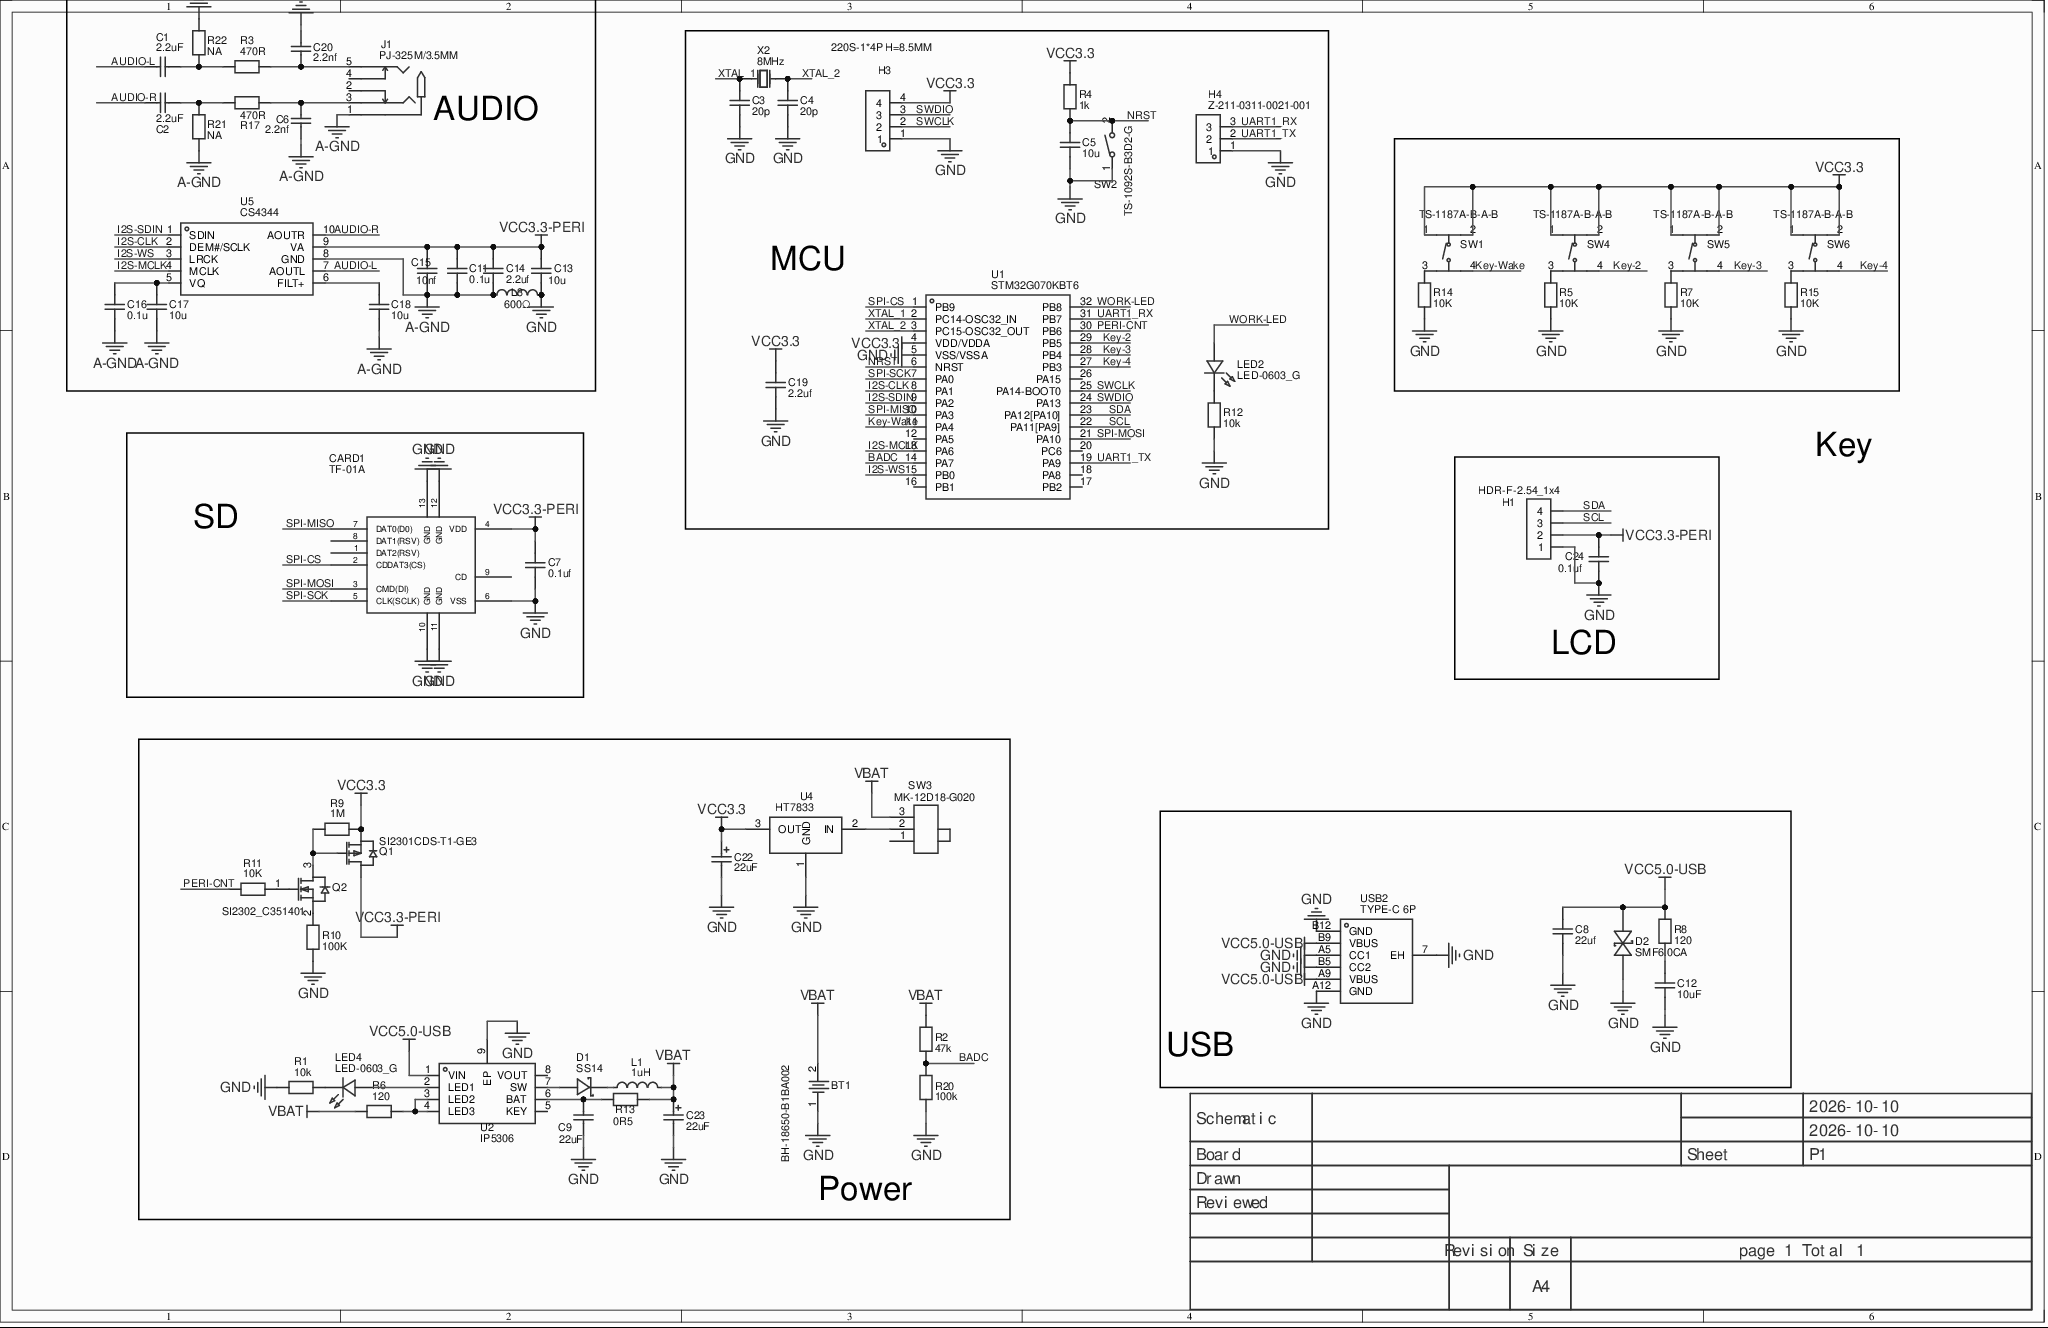
[diagram p0: MISC82317-2.schdoc]
# Altium schematic sheet MISC82317-2.schdoc
size 432 x 279 mm; Version: V1.0; @Project Name: MISC82317; @Update Date: 2026-10-10; @Create Date: 2026-10-10; @Board Name: MISC82317; @Create Time: 16:29:33; @Page Count: 1; @Page No: 1; @Schematic Name: MISC82317; @Update Time: 16:29:33; Size: A4

## Parts
BT1  BH-18650-B1BA002  [BATTERY-SMD_18650-1S-L77.1-W20.7-1]
C1  2.2uF  [C0603]
C2  2.2uF  [C0603]
C3  20p  [C0603]
C4  20p  [C0603]
C5  10u  [C0603]
C6  2.2nf  [C0603]
C7  0.1uf  [C0603]
C8  22uf  [C0603]
C9  22uF  [C0603]
C11  0.1u  [C0603]
C12  10uF  [C0603]
C13  10u  [C0603]
C14  2.2uf  [C0603]
C15  10nf  [C0603]
C16  0.1u  [C0603]
C17  10u  [C0603]
C18  10u  [C0603]
C19  2.2uf  [C0603]
C20  2.2nf  [C0603]
C22  22uF  [CAP-SMD_L3.5-W2.8-R-RD]
C23  22uF  [CAP-SMD_L3.5-W2.8-R-RD]
C24  0.1uf  [C0603]
CARD1  TF-01A  [TF-SMD_TF-01A]
D1  SS14  [SMA_L4.2-W2.6-LS5.3-RD]
D2  SMF6.0CA  [SOD-123FL_L2.8-W1.8-LS3.7-BI]
H1  HDR-F-2.54_1x4  [HDR-F-2.54_1X4]
H3  220S-1*4P H=8.5MM  [HDR-TH_4P-P2.54-V-F]
H4  Z-211-0311-0021-001  [HDR-TH_3P-P2.54-V-M-1]
J1  PJ-325M/3.5MM  [AUDIO-TH_PJ-325C]
L1  1uH  [IND-SMD_L6.8-W6.8_SMMS0630]
L3  600Ω  [L1206]
LED2  LED-0603_G  [LED0603_GREEN]
LED4  LED-0603_G  [LED0603_GREEN]
Q1  SI2301CDS-T1-GE3  [SOT-23-3_L3.0-W1.7-P0.95-LS2.9-BR]
Q2  SI2302_C351401  [SOT-23-3_L2.9-W1.3-P1.90-LS2.4]
R1  10k  [R0603]
R2  47k  [R0603]
R3  470R  [R0603]
R4  1k  [R0603]
R5  10K  [R0603]
R6  120  [R0603]
R7  10K  [R0603]
R8  120  [R0603]
R9  1M  [R0603]
R10  100K  [R0603]
R11  10K  [R0603]
R12  10k  [R0603]
R13  0R5  [R1206]
R14  10K  [R0603]
R15  10K  [R0603]
R17  470R  [R0603]
R20  100k  [R0603]
R21  NA  [R0603]
R22  NA  [R0603]
SW1  TS-1187A-B-A-B  [SW-SMD_4P-L5.1-W5.1-P3.70-LS6.5-TL-2]
SW2  TS-1092S-B3D2-G  [SW-SMD_L6.1-W3.6-LS7.9]
SW3  MK-12D18-G020  [SW-TH_MK-12D18-G040]
SW4  TS-1187A-B-A-B  [SW-SMD_4P-L5.1-W5.1-P3.70-LS6.5-TL-2]
SW5  TS-1187A-B-A-B  [SW-SMD_4P-L5.1-W5.1-P3.70-LS6.5-TL-2]
SW6  TS-1187A-B-A-B  [SW-SMD_4P-L5.1-W5.1-P3.70-LS6.5-TL-2]
U1  STM32G070KBT6  [LQFP-32_L7.0-W7.0-P0.80-LS9.0-BL]
U2  IP5306  [ESOP-8_L4.9-W3.9-P1.27-LS6.0-BL-EP]
U4  HT7833  [SOT-89_L4.5-W2.5-P1.50-LS4.2-BR]
U5  CS4344  [TSSOP-10_L3.0-W3.0-P0.50-LS4.9-BL]
USB2  TYPE-C 6P  [TYPE-C-SMD_TYPE-C-6P]
X2  8MHz  [CRYSTAL-SMD_L5.0-W3.2]

## Blocks framed on the sheet
AUDIO: C1 C2 C6 C11 C13-C18 C20 J1 L3 R3 R17 R21 R22 U5
MCU: C3-C5 C19 H3 H4 LED2 R4 R12 SW2 U1 X2
SD: C7 CARD1
LCD: C24 H1
Power: BT1 C9 C22 C23 D1 L1 LED4 Q1 Q2 R1 R2 R6 R9-R11 R13 R20 SW3 U2 U4
USB: C8 C12 D2 R8 USB2

## Nets
A-GND: C6.1 C11.1 C14.1 C15.1 C16.1 C17.1 C18.1 C20.2 J1.1 L3.1 R21.2 R22.1 U5.8(GND)
GND: BT1.1 C3.1 C4.1 C5.1 C7.1 C8.1 C9.1 C12.1 C13.1 C19.1 C22.2 C23.2 C24.1 CARD1.6(VSS) CARD1.10(GND) CARD1.11(GND) CARD1.12(GND) CARD1.13(GND) D2.1 H1.1 H3.1 H4.1 L3.2 R1.2 R5.1 R7.1 R10.2 R12.1 R14.1 R15.1 R20.1 SW2.1 U1.5(VSS/VSSA) U2.9(EP) U4.1(GND) USB2.7(EH) USB2.A5(CC1) USB2.A12(GND) USB2.B5(CC2) USB2.B12(GND)
VBAT: BT1.2 C23.1 L1.2 R2.2 R6.2 R13.2 SW3.3
VCC3.3: C19.2 C22.1 H3.4 Q1.2(S) R4.2 R9.1 SW1.1(A) SW1.2(B) SW4.1(A) SW4.2(B) SW5.1(A) SW5.2(B) SW6.1(A) SW6.2(B) U1.4(VDD/VDDA) U4.3(OUT)
VCC3.3-PERI: C7.2 C11.2 C13.2 C14.2 C15.2 C24.2 CARD1.4(VDD) H1.2 Q1.3(D) U5.9(VA)
VCC5.0-USB: C8.2 D2.2 R8.1 U2.1(VIN) USB2.A9(VBUS) USB2.B9(VBUS)
AUDIO-L: C1.1 U5.7(AOUTL)
AUDIO-R: C2.1 U5.10(AOUTR)
BADC: R2.1 R20.2 U1.14(PA7)
I2S-CLK: U1.8(PA1) U5.2(DEM#/SCLK)
I2S-MCLK: U1.13(PA6) U5.4(MCLK)
I2S-SDIN: U1.9(PA2) U5.1(SDIN)
I2S-WS: U1.15(PB0) U5.3(LRCK)
Key-2: SW4.4(D) U1.29(PB5)
Key-3: SW5.4(D) U1.28(PB4)
Key-4: SW6.4(D) U1.27(PB3)
Key-Wake: SW1.4(D) U1.11(PA4)
NRST: C5.2 R4.1 SW2.2 U1.6(NRST)
PERI-CNT: R11.1 U1.30(PB6)
SCL: H1.3 U1.22(PA11[PA9])
SDA: H1.4 U1.23(PA12[PA10])
SPI-CS: CARD1.2(CDDAT3(CS)) U1.1(PB9)
SPI-MISO: CARD1.7(DAT0(D0)) U1.10(PA3)
SPI-MOSI: CARD1.3(CMD(DI)) U1.21(PA10)
SPI-SCK: CARD1.5(CLK(SCLK)) U1.7(PA0)
SWCLK: H3.2 U1.25(PA14-BOOT0)
SWDIO: H3.3 U1.24(PA13)
UART1_RX: H4.3 U1.31(PB7)
UART1_TX: H4.2 U1.19(PA9)
WORK-LED: LED2.1 U1.32(PB8)
XTAL_1: C3.2 U1.2(PC14-OSC32_IN) X2.1(OSC1)
XTAL_2: C4.2 U1.3(PC15-OSC32_OUT) X2.2(OSC2)
NetC1_2: C1.2 R3.2 R22.2
NetC2_2: C2.2 R17.2 R21.1
NetC6_2: C6.2 J1.3 R17.1
NetC9_2: C9.2 R13.1 U2.6(BAT)
NetC12_2: C12.2 R8.2
NetC16_2: C16.2 C17.2 U5.5(VQ)
NetC18_2: C18.2 U5.6(FILT+)
NetC20_1: C20.1 J1.5 R3.1
NetD1_1: D1.1(K) L1.1
NetD1_2: D1.2(A) U2.7(SW)
NetLED2_2: LED2.2 R12.2
NetLED4_1: LED4.1 U2.2(LED1)
NetLED4_2: LED4.2 R1.1
NetQ1_1: Q1.1(G) Q2.3(D) R9.2
NetQ2_1: Q2.1(G) R11.2
NetQ2_2: Q2.2(S) R10.1
NetR5_2: R5.2 SW4.3(C)
NetR6_1: R6.1 U2.3(LED2) U2.4(LED3)
NetR7_2: R7.2 SW5.3(C)
NetR14_2: R14.2 SW1.3(C)
NetR15_2: R15.2 SW6.3(C)
NetSW3_2: SW3.2 U4.2(IN)

Not connected (* = marked no-connect by the designer): CARD1 1(DAT2(RSV))* 8(DAT1(RSV))* 9(CD)*; J1 2* 4*; SW3 1*; U1 12(PA5)* 16(PB1)* 17(PB2)* 18(PA8)* 20(PC6)* 26(PA15)*; U2 5(KEY)* 8(VOUT)*

## Notes on the sheet
- Key
- 2026-10-10
- Schematic
- Board
- Sheet
- P1
- Drawn
- Reviewed
- Revision
- Size
- A4
- page 1 Total 1

## Library data of the parts
BT1 = BH-18650-B1BA002: Manufacturer: MYOUNG(美阳); Add into BOM: yes; 3D Model: 6c4af93ff24747e7be32603ea977d5150819f05c4eef4c71ace90d822a990e87; Symbol: BH-18650-B1BA002; Device: BH-18650-B1BA002; Convert to PCB: yes; Supplier: LCSC; Supplier Part: C2988620; Manufacturer Part: BH-18650-B1BA002; link: https://atta.szlcsc.com/upload/public/pdf/source/20220402/870DB99AB50CA0DF8D51CF7C86A51FAB.pdf; JLCPCB Part Class: Extended Part; Origin Footprint: BATTERY-SMD_18650-1S-L77.1-W20.7-1; FootprintName: BATTERY-SMD_18650-1S-L77.1-W20.7-1; ModelName: BATTERY-SMD_18650-1S-L77.1-W20.7-1
C1 C2 C6 C20 = CL10A225KO8NNNC: Manufacturer: SAMSUNG; Add into BOM: yes; 3D Model: fca5be93b99f4b5a9a2fd372d58c31d90819f05c4eef4c71ace90d822a990e87; Device: CL10A225KO8NNNC; Convert to PCB: yes; Supplier: LCSC; Manufacturer Part: CL10A225KO8NNNC; Supplier Part: C23630; JLCPCB Part Class: Basic Part; Origin Footprint: C0603; FootprintName: C0603; ModelName: C0603
  C1 C2: Symbol: 2.2uF
  C6 C20: Symbol: 2.2nf
C3 C4 = 20p: Add into BOM: yes; 3D Model: fca5be93b99f4b5a9a2fd372d58c31d90819f05c4eef4c71ace90d822a990e87; Symbol: 20p; Device: 20p; Convert to PCB: yes; Origin Footprint: C0603; FootprintName: C0603; ModelName: C0603
C5 C13 C17 C18 = 10u: Add into BOM: yes; 3D Model: fca5be93b99f4b5a9a2fd372d58c31d90819f05c4eef4c71ace90d822a990e87; Symbol: 10u; Device: 10u; Convert to PCB: yes; Origin Footprint: C0603; FootprintName: C0603; ModelName: C0603
C7 C24 = 0.1uf: Add into BOM: yes; 3D Model: fca5be93b99f4b5a9a2fd372d58c31d90819f05c4eef4c71ace90d822a990e87; Symbol: 0.1uf; Device: 0.1uf; Convert to PCB: yes; Origin Footprint: C0603; FootprintName: C0603; ModelName: C0603
C8 C12 = 0603X106M250NT: Manufacturer: FH(Guangdong Fenghua Advanced Tech); Add into BOM: yes; 3D Model: fca5be93b99f4b5a9a2fd372d58c31d90819f05c4eef4c71ace90d822a990e87; Device: 0603X106M250NT; Convert to PCB: yes; Supplier: LCSC; Supplier Part: C479655; Manufacturer Part: 0603X106M250NT; JLCPCB Part Class: Extended Part; Origin Footprint: C0603; FootprintName: C0603; ModelName: C0603
  C8: Symbol: 22uf
  C12: Symbol: 10uF
C9 = CC0603MRX5R5BB226: Manufacturer: YAGEO; Add into BOM: yes; 3D Model: fca5be93b99f4b5a9a2fd372d58c31d90819f05c4eef4c71ace90d822a990e87; Symbol: 22uF; Device: CC0603MRX5R5BB226; Convert to PCB: yes; Supplier: LCSC; Manufacturer Part: CC0603MRX5R5BB226; Supplier Part: C109448; JLCPCB Part Class: Extended Part; Origin Footprint: C0603; FootprintName: C0603; ModelName: C0603
C11 C16 = 0.1u: Add into BOM: yes; 3D Model: fca5be93b99f4b5a9a2fd372d58c31d90819f05c4eef4c71ace90d822a990e87; Symbol: 0.1u; Device: 0.1u; Convert to PCB: yes; Origin Footprint: C0603; FootprintName: C0603; ModelName: C0603
C14 C19 = 2.2uf: Add into BOM: yes; 3D Model: fca5be93b99f4b5a9a2fd372d58c31d90819f05c4eef4c71ace90d822a990e87; Symbol: 2.2uf; Device: 2.2uf; Convert to PCB: yes; Origin Footprint: C0603; FootprintName: C0603; ModelName: C0603
C15 = 10nf: Add into BOM: yes; 3D Model: fca5be93b99f4b5a9a2fd372d58c31d90819f05c4eef4c71ace90d822a990e87; Symbol: 10nf; Device: 10nf; Convert to PCB: yes; Origin Footprint: C0603; FootprintName: C0603; ModelName: C0603
C22 C23 = TAJB226K016RNJ: Manufacturer: AVX; Add into BOM: yes; Symbol: 22uF; Device: TAJB226K016RNJ; Convert to PCB: yes; Supplier: LCSC; Manufacturer Part: TAJB226K016RNJ; Supplier Part: C8020; JLCPCB Part Class: Extended Part; Origin Footprint: CAP-SMD_L3.5-W2.8-R-RD; FootprintName: CAP-SMD_L3.5-W2.8-R-RD
CARD1 = TF-01A: Manufacturer: HRO; Add into BOM: yes; 3D Model: 2d64e7db065c4e679bbb440594759bbc0819f05c4eef4c71ace90d822a990e87; Symbol: TF-01A; Device: TF-01A; Convert to PCB: yes; Supplier: LCSC; Manufacturer Part: TF-01A; Supplier Part: C91145; JLCPCB Part Class: Extended Part; Origin Footprint: TF-SMD_TF-01A; FootprintName: TF-SMD_TF-01A; ModelName: TF-SMD_TF-01A
D1 = SS14: Manufacturer: MDD; Add into BOM: yes; 3D Model: c9e8185d46a94015b9fa58a531b156cf0819f05c4eef4c71ace90d822a990e87; Symbol: SS14; Device: SS14; Convert to PCB: yes; Supplier: LCSC; Manufacturer Part: SS14; Supplier Part: C2480; JLCPCB Part Class: Basic Part; Origin Footprint: SMA_L4.2-W2.6-LS5.3-RD; FootprintName: SMA_L4.2-W2.6-LS5.3-RD; ModelName: SMA_L4.2-W2.6-LS5.3-RD
D2 = SMF6.0CA: Manufacturer: MDD; Add into BOM: yes; 3D Model: d105299b3871451c86f679efef28ff8f0819f05c4eef4c71ace90d822a990e87; Symbol: SMF6.0CA; Device: SMF6.0CA; Convert to PCB: yes; Supplier: LCSC; Manufacturer Part: SMF6.0CA; Supplier Part: C123791; JLCPCB Part Class: Extended Part; Origin Footprint: SOD-123FL_L2.8-W1.8-LS3.7-BI; FootprintName: SOD-123FL_L2.8-W1.8-LS3.7-BI; ModelName: SOD-123FL_L2.8-W1.8-LS3.7-BI
H1 = HDR-F-2.54_1x4: Add into BOM: yes; 3D Model: f101a8d78d1e4ea1b9dbaf5a3cdaf2060819f05c4eef4c71ace90d822a990e87; Symbol: HDR-F-2.54_1x4; Device: HDR-F-2.54_1x4; Convert to PCB: yes; Supplier Part: C225501; Supplier: LCSC; Origin Footprint: HDR-F-2.54_1X4; FootprintName: HDR-F-2.54_1X4; ModelName: HDR-F-2.54_1x4
H3 = 220S-1*4P H=8.5MM Ytype Gold-plated: Manufacturer: Ckmtw; Add into BOM: yes; 3D Model: d187812051054f85879fcaa51a310d8e0819f05c4eef4c71ace90d822a990e87; Symbol: 220S-1*4P H=8.5MM; Device: 220S-1*4P H=8.5MM Ytype Gold-plated; Convert to PCB: yes; Supplier: LCSC; Manufacturer Part: 220S-1*4P H=8.5MM Ytype Gold-plated; Supplier Part: C124413; JLCPCB Part Class: Extended Part; Origin Footprint: HDR-TH_4P-P2.54-V-F; FootprintName: HDR-TH_4P-P2.54-V-F; ModelName: HDR-TH_4P-P2.54-V-F
H4 = Z-211-0311-0021-001: Manufacturer: ZHENGLING; Add into BOM: yes; Symbol: Z-211-0311-0021-001; Device: Z-211-0311-0021-001; Convert to PCB: yes; Supplier: LCSC; Manufacturer Part: Z-211-0311-0021-001; Supplier Part: C152153; JLCPCB Part Class: Extended Part; Origin Footprint: HDR-TH_3P-P2.54-V-M-1; FootprintName: HDR-TH_3P-P2.54-V-M-1
J1 = PJ-325M/3.5MM: Manufacturer: BOOMELE; Add into BOM: yes; 3D Model: 332d8d5c7f544556a9ac40ab7a6b8b0c0819f05c4eef4c71ace90d822a990e87; Symbol: PJ-325M/3.5MM; Device: PJ-325M/3.5MM; Convert to PCB: yes; Supplier: LCSC; Manufacturer Part: PJ-325M/3.5MM; Supplier Part: C26230; JLCPCB Part Class: Extended Part; Origin Footprint: AUDIO-TH_PJ-325C; FootprintName: AUDIO-TH_PJ-325C; ModelName: AUDIO-TH_PJ-325C
L1 = SMMS0630-1R0M: Manufacturer: SXN; Add into BOM: yes; Symbol: 1uH; Device: SMMS0630-1R0M; Convert to PCB: yes; Supplier: LCSC; Manufacturer Part: SMMS0630-1R0M; Supplier Part: C128684; JLCPCB Part Class: Extended Part; Origin Footprint: IND-SMD_L6.8-W6.8_SMMS0630; FootprintName: IND-SMD_L6.8-W6.8_SMMS0630
L3 = CBW321609U601T: Manufacturer: FH; Add into BOM: yes; Symbol: 600Ω; Device: CBW321609U601T; Convert to PCB: yes; Supplier: LCSC; Manufacturer Part: CBW321609U601T; Supplier Part: C73732; JLCPCB Part Class: Extended Part; Origin Footprint: L1206; FootprintName: L1206
LED2 LED4 = 19-217/GHC-YR1S2/3T: Manufacturer: EVERLIGHT(台湾亿光); Add into BOM: yes; Symbol: LED-0603_G; Device: 19-217/GHC-YR1S2/3T; Convert to PCB: yes; Manufacturer Part: 19-217/GHC-YR1S2/3T; Supplier Part: C72043; Supplier: LCSC; Origin Footprint: LED0603_GREEN; FootprintName: LED0603_GREEN
Q1 = SI2301CDS-T1-GE3: Manufacturer: VISHAY; Add into BOM: yes; Symbol: SI2301CDS-T1-GE3; Device: SI2301CDS-T1-GE3; Convert to PCB: yes; Supplier: LCSC; Manufacturer Part: SI2301CDS-T1-GE3; Supplier Part: C10487; JLCPCB Part Class: Basic Part; Origin Footprint: SOT-23-3_L3.0-W1.7-P0.95-LS2.9-BR; FootprintName: SOT-23-3_L3.0-W1.7-P0.95-LS2.9-BR
Q2 = SI2302: Manufacturer: PUOLOP; Add into BOM: yes; 3D Model: 115ef394a879442d90491e61279301380819f05c4eef4c71ace90d822a990e87; Symbol: SI2302_C351401; Device: SI2302; Convert to PCB: yes; Supplier: LCSC; Supplier Part: C351401; Manufacturer Part: SI2302; JLCPCB Part Class: Extended Part; Origin Footprint: SOT-23-3_L2.9-W1.3-P1.90-LS2.4; FootprintName: SOT-23-3_L2.9-W1.3-P1.90-LS2.4; ModelName: SOT-23-3_L2.9-W1.3-P1.90-LS2.4
R1 R12 = 10k: Add into BOM: yes; 3D Model: fc143cca1e79419f9cd78b61e9279f080819f05c4eef4c71ace90d822a990e87; Symbol: 10k; Device: 10k; Convert to PCB: yes; Origin Footprint: R0603; FootprintName: R0603; ModelName: R0603
R2 = 47k: Add into BOM: yes; 3D Model: fc143cca1e79419f9cd78b61e9279f080819f05c4eef4c71ace90d822a990e87; Symbol: 47k; Device: 47k; Convert to PCB: yes; Origin Footprint: R0603; FootprintName: R0603; ModelName: R0603
R3 R17 = 470R: Add into BOM: yes; 3D Model: fc143cca1e79419f9cd78b61e9279f080819f05c4eef4c71ace90d822a990e87; Symbol: 470R; Device: 470R; Convert to PCB: yes; Origin Footprint: R0603; FootprintName: R0603; ModelName: R0603
R4 = 1k: Add into BOM: yes; 3D Model: fc143cca1e79419f9cd78b61e9279f080819f05c4eef4c71ace90d822a990e87; Symbol: 1k; Device: 1k; Convert to PCB: yes; Origin Footprint: R0603; FootprintName: R0603; ModelName: R0603
R5 R7 R11 R14 R15 = 10K: Add into BOM: yes; 3D Model: fc143cca1e79419f9cd78b61e9279f080819f05c4eef4c71ace90d822a990e87; Symbol: 10K; Device: 10K; Convert to PCB: yes; Origin Footprint: R0603; FootprintName: R0603; ModelName: R0603
R6 R8 = 120: Add into BOM: yes; 3D Model: fc143cca1e79419f9cd78b61e9279f080819f05c4eef4c71ace90d822a990e87; Symbol: 120; Device: 120; Convert to PCB: yes; Origin Footprint: R0603; FootprintName: R0603; ModelName: R0603
R9 = 1M: Add into BOM: yes; 3D Model: fc143cca1e79419f9cd78b61e9279f080819f05c4eef4c71ace90d822a990e87; Symbol: 1M; Device: 1M; Convert to PCB: yes; Origin Footprint: R0603; FootprintName: R0603; ModelName: R0603
R10 = 100K: Add into BOM: yes; 3D Model: fc143cca1e79419f9cd78b61e9279f080819f05c4eef4c71ace90d822a990e87; Symbol: 100K; Device: 100K; Convert to PCB: yes; Origin Footprint: R0603; FootprintName: R0603; ModelName: R0603
R13 = 1206W4F590LT5E: Manufacturer: UNI-ROYAL(Uniroyal Elec); Add into BOM: yes; Resistance (Ohms): 0.59; Symbol: 0R5; Device: 1206W4F590LT5E; Convert to PCB: yes; Supplier: LCSC; Supplier Part: C473018; Manufacturer Part: 1206W4F590LT5E; JLCPCB Part Class: Extended Part; Origin Footprint: R1206; FootprintName: R1206
R20 = 100k: Add into BOM: yes; 3D Model: fc143cca1e79419f9cd78b61e9279f080819f05c4eef4c71ace90d822a990e87; Symbol: 100k; Device: 100k; Convert to PCB: yes; Origin Footprint: R0603; FootprintName: R0603; ModelName: R0603
R21 R22 = NA: Add into BOM: yes; 3D Model: fc143cca1e79419f9cd78b61e9279f080819f05c4eef4c71ace90d822a990e87; Symbol: NA; Device: NA; Convert to PCB: yes; Origin Footprint: R0603; FootprintName: R0603; ModelName: R0603
SW1 SW4-SW6 = TS-1187A-B-A-B: Manufacturer: XKB Enterprise; Add into BOM: yes; Symbol: TS-1187A-B-A-B; Device: TS-1187A-B-A-B; Convert to PCB: yes; Supplier: LCSC; Supplier Part: C318884; Manufacturer Part: TS-1187A-B-A-B; JLCPCB Part Class: Basic Part; Origin Footprint: SW-SMD_4P-L5.1-W5.1-P3.70-LS6.5-TL-2; FootprintName: SW-SMD_4P-L5.1-W5.1-P3.70-LS6.5-TL-2
SW2 = TS-1092S-B3D2-G: Manufacturer: Yuandi; Add into BOM: yes; Symbol: TS-1092S-B3D2-G; Device: TS-1092S-B3D2-G; Convert to PCB: yes; Supplier: LCSC; Supplier Part: C520860; Manufacturer Part: TS-1092S-B3D2-G; JLCPCB Part Class: Extended Part; Origin Footprint: SW-SMD_L6.1-W3.6-LS7.9; FootprintName: SW-SMD_L6.1-W3.6-LS7.9
SW3 = MK-12D18-G020: Manufacturer: G-Switch(品赞); Add into BOM: yes; 3D Model: 10e91de5902f4d769c8626292907b3900819f05c4eef4c71ace90d822a990e87; Symbol: MK-12D18-G020; Device: MK-12D18-G020; Convert to PCB: yes; Supplier: LCSC; Supplier Part: C3019727; Manufacturer Part: MK-12D18-G020; link: https://atta.szlcsc.com/upload/public/pdf/source/20201201/C963202_825FB742C5BA766BED52E1DDA96DE5A3.pdf; Origin Footprint: SW-TH_MK-12D18-G040; FootprintName: SW-TH_MK-12D18-G040; ModelName: SW-TH_MK-12D18-G040
U1 = STM32G070KBT6: Manufacturer: STMicroelectronics; Add into BOM: yes; Symbol: STM32G070KBT6; Device: STM32G070KBT6; Convert to PCB: yes; Supplier: LCSC; Supplier Part: C529339; Manufacturer Part: STM32G070KBT6; JLCPCB Part Class: Extended Part; Origin Footprint: LQFP-32_L7.0-W7.0-P0.80-LS9.0-BL; FootprintName: LQFP-32_L7.0-W7.0-P0.80-LS9.0-BL
U2 = IP5306: Manufacturer: INJOINIC; Add into BOM: yes; Symbol: IP5306; Device: IP5306; Convert to PCB: yes; Supplier: LCSC; Supplier Part: C181692; Manufacturer Part: IP5306; JLCPCB Part Class: Extended Part; Origin Footprint: ESOP-8_L4.9-W3.9-P1.27-LS6.0-BL-EP; FootprintName: ESOP-8_L4.9-W3.9-P1.27-LS6.0-BL-EP
U4 = HT7833: Manufacturer: HOLTEK; Add into BOM: yes; Symbol: HT7833; Device: HT7833; Convert to PCB: yes; Supplier: LCSC; Manufacturer Part: HT7833; Supplier Part: C50936; JLCPCB Part Class: Extended Part; Origin Footprint: SOT-89_L4.5-W2.5-P1.50-LS4.2-BR; FootprintName: SOT-89_L4.5-W2.5-P1.50-LS4.2-BR
U5 = CS4344: Manufacturer: null; Add into BOM: yes; Symbol: CS4344; Device: CS4344; Convert to PCB: yes; Supplier: LCSC; Supplier Part: C2914311; Manufacturer Part: CS4344; JLCPCB Part Class: Extended Part; Origin Footprint: TSSOP-10_L3.0-W3.0-P0.50-LS4.9-BL; FootprintName: TSSOP-10_L3.0-W3.0-P0.50-LS4.9-BL
USB2 = TYPE-C 6P: Manufacturer: SHOU HAN; Add into BOM: yes; Symbol: TYPE-C 6P; Device: TYPE-C 6P; Convert to PCB: yes; Supplier: LCSC; Supplier Part: C456012; Manufacturer Part: TYPE-C 6P; JLCPCB Part Class: Extended Part; Origin Footprint: TYPE-C-SMD_TYPE-C-6P; FootprintName: TYPE-C-SMD_TYPE-C-6P
X2 = X50328MSB2GI: Manufacturer: YXC; Add into BOM: yes; 3D Model: d7c39c66443246ff83c2003c1e1eb6f10819f05c4eef4c71ace90d822a990e87; Symbol: 8MHz; Device: X50328MSB2GI; Convert to PCB: yes; Supplier: LCSC; Manufacturer Part: X50328MSB2GI; Supplier Part: C115962; JLCPCB Part Class: Basic Part; Origin Footprint: CRYSTAL-SMD_L5.0-W3.2; FootprintName: CRYSTAL-SMD_L5.0-W3.2; ModelName: CRYSTAL-SMD_L5.0-W3.2